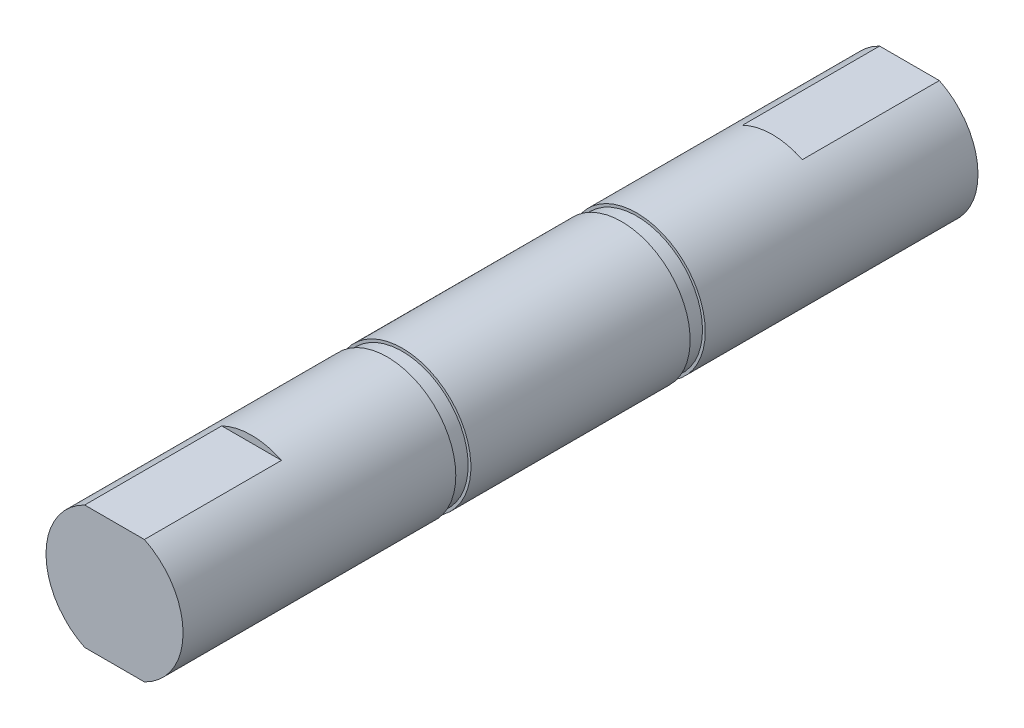
from build123d import *

# Parameters (mm, degrees)
SKETCH_1_R          = 5
EXTRUDE_1_DEPTH     = 29
CUT_EXTRUDE_START   = 1.1
SKETCH_3_R          = 5
SKETCH_3_R_2        = 4.8
CUT_EXTRUDE_2_DEPTH = 1.1
CUT_EXTRUDE_1_DEPTH = 10


with BuildPart() as part:
    # 草图1 → 凸台-拉伸1 (new, symmetric)
    with BuildSketch(Plane.XY):
        with Locations(Location((0, 0, 0), (0, 0, 180))):
            Circle(SKETCH_1_R)
    extrude(amount=EXTRUDE_1_DEPTH, both=True)

    # 草图3 → 切除-拉伸2 (cut)
    with BuildSketch(Plane.XY.offset(8).offset(CUT_EXTRUDE_START)):
        with Locations(Location((0, 0, 0), (0, 0, 180))):
            Circle(SKETCH_3_R)
        Circle(SKETCH_3_R_2, mode=Mode.SUBTRACT)
    cut_extrude_2 = extrude(amount=-CUT_EXTRUDE_2_DEPTH, mode=Mode.SUBTRACT)

    # 镜向2: 切除-拉伸2 across plane
    add(cut_extrude_2.mirror(Plane.XY), mode=Mode.SUBTRACT)

    # 草图2 → 切除-拉伸1 (cut)
    with BuildSketch(Plane.XY.offset(29)):
        with BuildLine():
            Line((-2.179449472, 4.5), (2.179449472, 4.5))
            ThreePointArc((2.179449472, 4.5), (0, 5), (-2.179449472, 4.5))
        make_face()
        with BuildLine():
            Line((-2.179449472, -4.5), (2.179449472, -4.5))
            ThreePointArc((2.179449472, -4.5), (0, -5), (-2.179449472, -4.5))
        make_face()
    cut_extrude_1 = extrude(amount=-CUT_EXTRUDE_1_DEPTH, mode=Mode.SUBTRACT)

    # 镜向1: 切除-拉伸1 across plane
    add(cut_extrude_1.mirror(Plane.XY), mode=Mode.SUBTRACT)


solid = part.part
